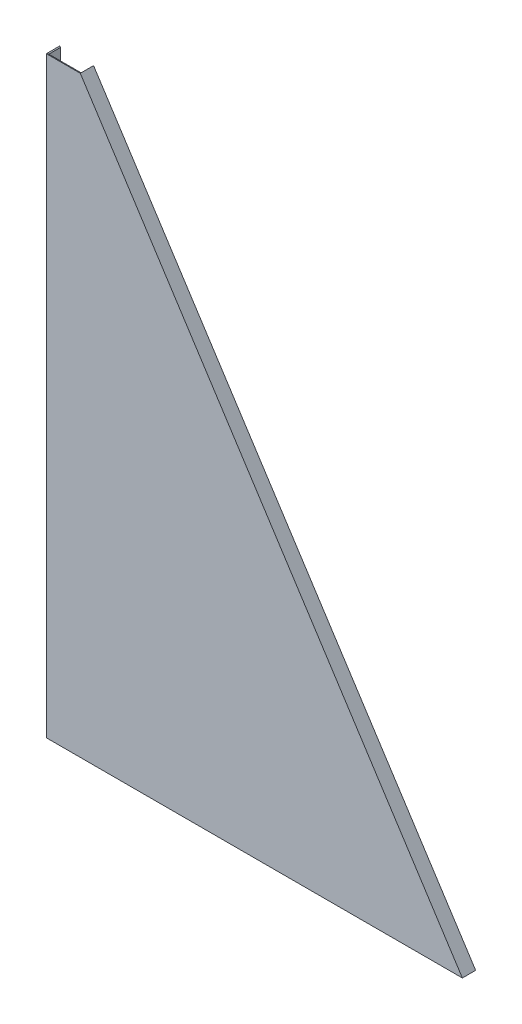
from build123d import *

# Parameters (mm, degrees)
SKETCH1_W           = 1002
SKETCH1_H           = 1427
BOSS_EXTRUDE1_DEPTH = 2
CUT_EXTRUDE1_DEPTH  = 2
BOSS_EXTRUDE2_DEPTH = 30


with BuildPart() as part:
    # Sketch1 → Boss-Extrude1 (new body)
    with BuildSketch(Plane.XY):
        Rectangle(SKETCH1_W, SKETCH1_H)
    extrude(amount=BOSS_EXTRUDE1_DEPTH)

    # Sketch2 → Cut-Extrude1 (cut)
    with BuildSketch(Plane.XY.offset(2)):
        Polygon((-419.25, 713.5), (501, -713.5), (501, 713.5), align=None)
    extrude(amount=-CUT_EXTRUDE1_DEPTH, mode=Mode.SUBTRACT)

    # Sketch4 → Boss-Extrude2 (add)
    with BuildSketch(Plane(origin=(0, 0, 0), x_dir=(-1, 0, 0), z_dir=(0, 0, -1))):
        Polygon((420.340042889, 711.5), (-497.33041962, -711.5), (499, -711.5), (499, 711.5), (501, 713.5), (501, -713.5), (-501, -713.5), (419.25, 713.5), align=None)
    extrude(amount=BOSS_EXTRUDE2_DEPTH)


solid = part.part
